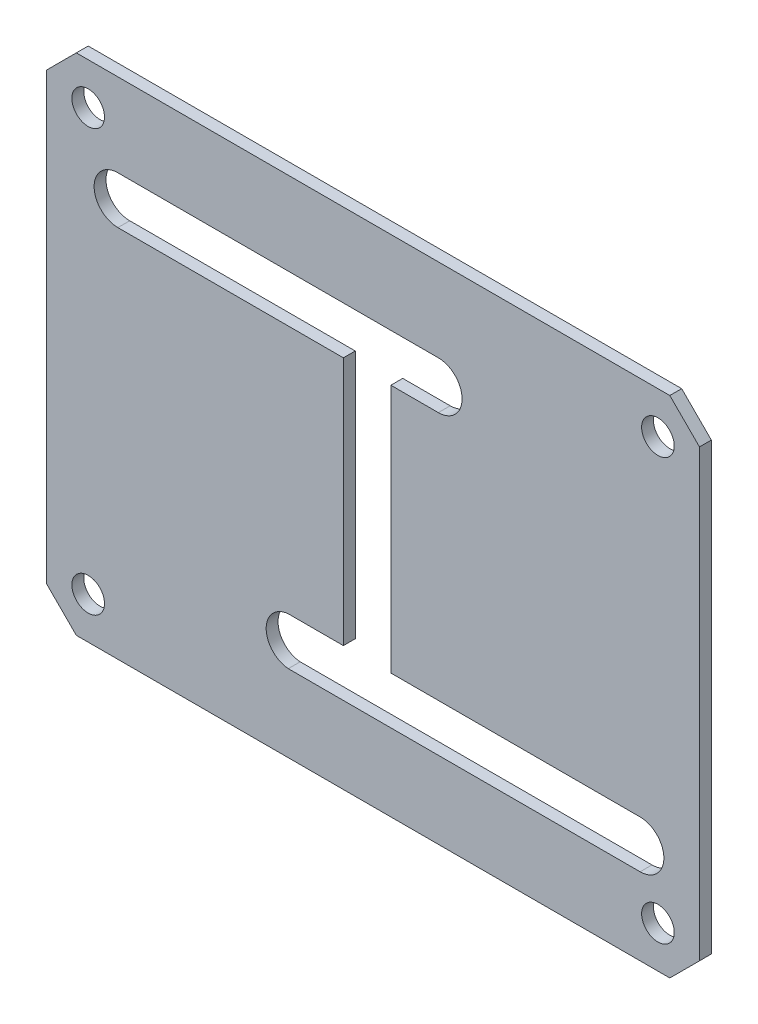
SolidWorks part; units mm, degrees
material "聚脂树脂"
ref_plane "前视基准面" through (0, 0, 0) normal (0, 0, 1) x (1, 0, 0)
ref_plane "上视基准面" through (0, 0, 0) normal (0, 1, 0) x (1, 0, 0)
ref_plane "右视基准面" through (0, 0, 0) normal (1, 0, 0) x (0, 0, -1)
sketch "草图1" plane through (0, 0, 0) normal (0, 0, 1) x (1, 0, 0)
  line L16 (357, 44.4275) -> (457, 44.4275)
  line L17 (457, 44.4275) -> (462, 49.4275)
  line L18 (462, 49.4275) -> (462, 124.4275)
  line L19 (462, 124.4275) -> (457, 129.4275)
  line L20 (457, 129.4275) -> (357, 129.4275)
  line L21 (357, 129.4275) -> (352, 124.4275)
  line L22 (352, 124.4275) -> (352, 49.4275)
  line L23 (352, 49.4275) -> (357, 44.4275)
extrude "凸台-拉伸1" add sketch "草图1" along normal blind 2
sketch "草图2" plane through (0, 0, 2) normal (0, 0, 1) x (1, 0, 0)
  line L0 (357, 44.4275) -> (457, 44.4275) construction
  line L1 (452, 57.4275) -> (392.7185, 57.4275)
  line L2 (462, 49.4275) -> (462, 124.4275) construction
  line L3 (452, 65.4275) -> (410, 65.4275)
  line L4 (410, 65.4275) -> (410, 107.4275)
  line L5 (418, 107.4275) -> (410, 107.4275)
  line L6 (402, 65.4275) -> (402, 107.4275)
  line L7 (418, 115.4275) -> (364, 115.4275)
  line L8 (402, 65.4275) -> (402, 107.4275) construction
  line L10 (402, 65.4275) -> (393.2815, 65.4275)
  line L11 (402, 107.4275) -> (364, 107.4275)
  line L13 (352, 124.4275) -> (352, 49.4275) construction
  arc A1 (452, 57.4275) -> (452, 65.4275) centre (452, 61.4275) ccw
  arc A2 (418, 107.4275) -> (418, 115.4275) centre (418, 111.4275) ccw
  arc A3 (364, 115.4275) -> (364, 107.4275) centre (364, 111.4275) ccw
  arc A4 (393.2815, 65.4275) -> (392.7185, 57.4275) centre (393, 61.4275) ccw
  dimension "D3" = 63
  dimension "D5" = 8
  dimension "D7" = 10
  dimension "D1" = 8
  dimension "D2" = 13
  dimension "D4" = 8
  dimension "D6" = 54
  dimension "D8" = 59
  dimension "D9" = 17
  dimension "D10" = 50
extrude "切除-拉伸1" cut sketch "草图2" against normal blind 2
sketch "草图3" plane through (0, 0, 2) normal (0, 0, 1) x (1, 0, 0)
  line L0 (352, 124.4275) -> (352, 49.4275) construction
  line L1 (457, 129.4275) -> (357, 129.4275) construction
  line L2 (357, 44.4275) -> (457, 44.4275) construction
  line L3 (462, 49.4275) -> (462, 124.4275) construction
  circle A0 centre (455, 51.4275) radius 2.75
  circle A1 centre (359, 51.4275) radius 2.75
  circle A2 centre (455, 122.4275) radius 2.75
  circle A3 centre (359, 122.4275) radius 2.75
  dimension "D1" = 5.5
  dimension "D4" = 7
  dimension "D2" = 7
  dimension "D3" = 7
  dimension "D5" = 7
extrude "切除-拉伸2" cut sketch "草图3" against normal blind 2
